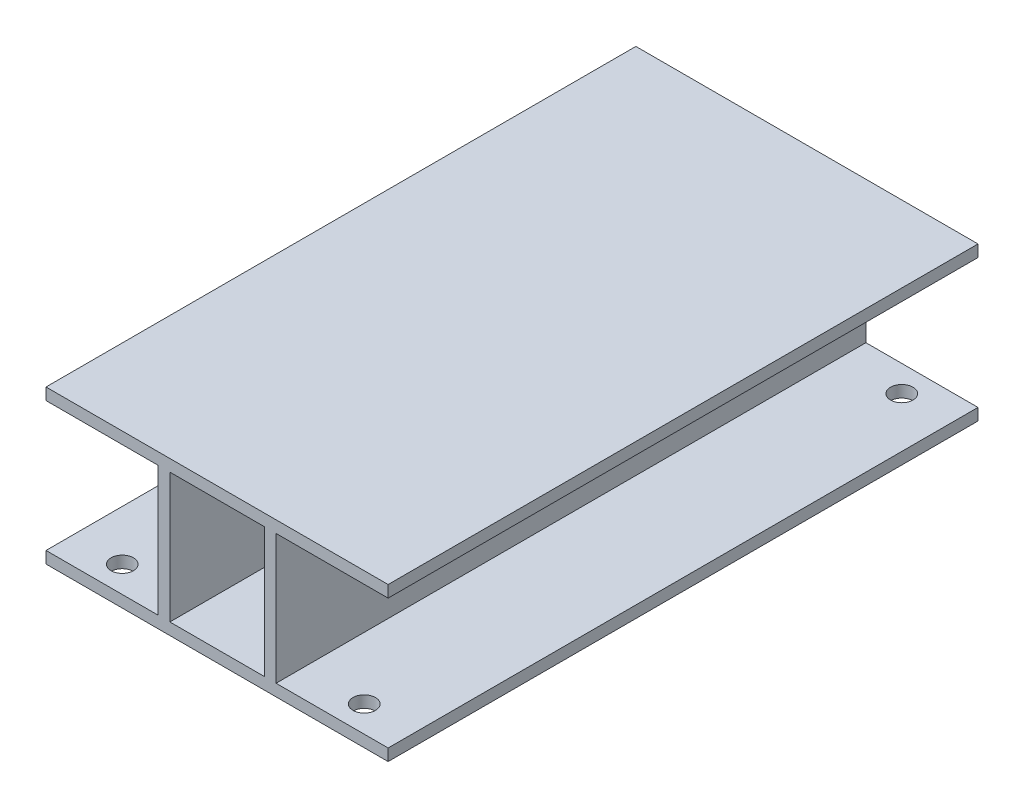
from build123d import *

# Parameters (mm, degrees)
SKETCH1_W           = 160
SKETCH1_H           = 220
BOSS_EXTRUDE1_DEPTH = 1000
SKETCH2_R           = 19
CUT_EXTRUDE1_DEPTH  = 30


with BuildPart() as part:
    # Sketch1 → Boss-Extrude1 (new body)
    with BuildSketch(Plane.XY):
        Polygon((-290, 260), (290, 260), (290, 240), (100, 240), (100, 20), (290, 20), (290, 0), (-290, 0), (-290, 20), (-100, 20), (-100, 240), (-290, 240), align=None)
        with Locations((0, 130)):
            Rectangle(SKETCH1_W, SKETCH1_H, mode=Mode.SUBTRACT)
    extrude(amount=BOSS_EXTRUDE1_DEPTH)

    # Sketch2 → Cut-Extrude1 (cut)
    with BuildSketch(Plane(origin=(0, 0, 0), x_dir=(-1, 0, 0), z_dir=(0, -1, 0))):
        with Locations(Location((205.124206689, -955.639521656, 0), (0, 0, 90))):
            Circle(SKETCH2_R)
        with Locations(Location((-205.124206689, -955.639521656, 0), (0, 0, 90))):
            Circle(SKETCH2_R)
        with Locations(Location((-205.124206689, -44.360478344, 0), (0, 0, 90))):
            Circle(SKETCH2_R)
        with Locations(Location((205.124206689, -44.360478344, 0), (0, 0, 90))):
            Circle(SKETCH2_R)
    extrude(amount=-CUT_EXTRUDE1_DEPTH, mode=Mode.SUBTRACT)


solid = part.part
